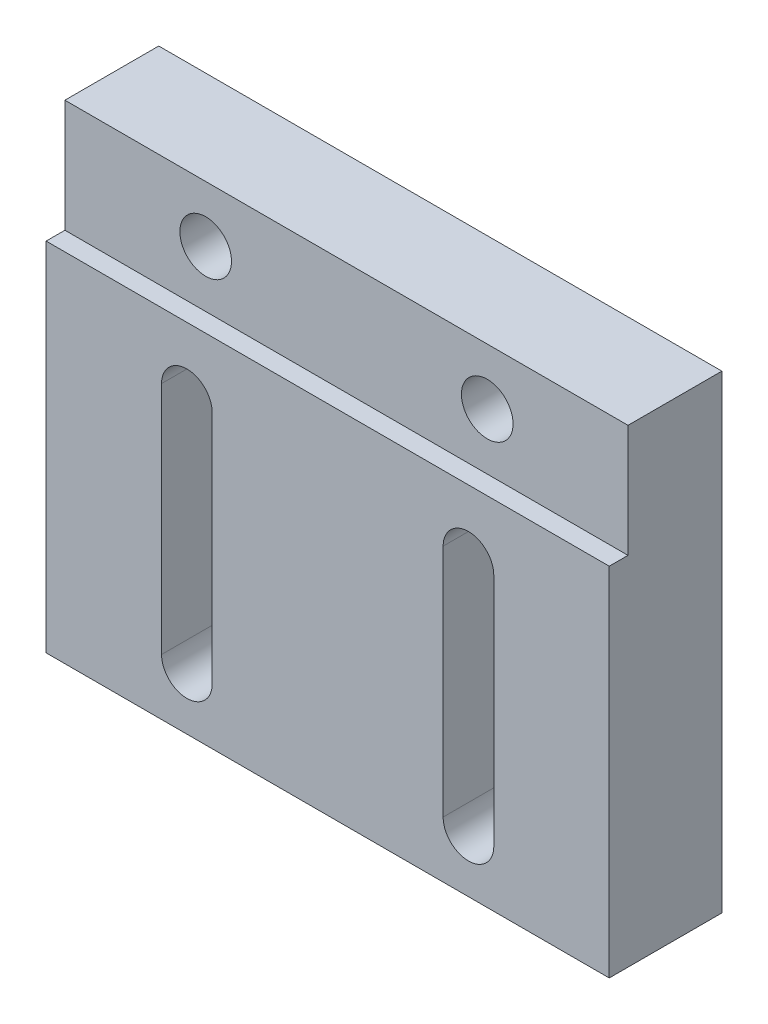
SolidWorks part; units mm, degrees
material "6061 合金"
ref_plane "前基準面" through (0, 0, 0) normal (0, 0, 1) x (1, 0, 0)
ref_plane "上基準面" through (0, 0, 0) normal (0, 1, 0) x (1, 0, 0)
ref_plane "右基準面" through (0, 0, 0) normal (1, 0, 0) x (0, 0, -1)
sketch "草图1" plane through (0, 0, 0) normal (0, 0, 1) x (1, 0, 0)
  line L1 (-30, 25) -> (30, 25)
  line L2 (-30, 25) -> (-30, -25)
  line L3 (-30, -25) -> (30, -25)
  line L4 (30, 25) -> (30, -25)
  line L5 (-30, 25) -> (30, -25) construction
  line L6 (-30, -25) -> (30, 25) construction
  point P0 (0, 0)
  dimension "D1" = 60
  dimension "D2" = 50
extrude "凸台-拉伸1" add sketch "草图1" along normal mid plane 12
sketch "草图2" plane through (0, 0, 6) normal (0, 0, 1) x (1, 0, 0)
  line L0 (30, -25) -> (30, 25) construction
  line L1 (-30, 25) -> (30, 25)
  line L2 (-30, 25) -> (-30, 13)
  line L3 (-30, 13) -> (30, 13)
  line L4 (30, 25) -> (30, 13)
  dimension "D1" = 12
extrude "切除-拉伸1" cut sketch "草图2" against normal blind 2
sketch "草图3" plane through (0, 0, 6) normal (0, 0, 1) x (1, 0, 0)
  line L0 (-15, -19) -> (-15, 6) construction
  line L1 (-17.7, -19) -> (-17.7, 6)
  line L2 (-12.3, -19) -> (-12.3, 6)
  line L3 (15, -19) -> (15, 6) construction
  line L4 (12.3, -19) -> (12.3, 6)
  line L5 (17.7, -19) -> (17.7, 6)
  line L6 (-15, -19) -> (15, -19) construction
  line L7 (0, -19) -> (0, -25) construction
  line L8 (-30, -25) -> (30, -25) construction
  arc A0 (-17.7, -19) -> (-12.3, -19) centre (-15, -19) ccw
  arc A1 (-12.3, 6) -> (-17.7, 6) centre (-15, 6) ccw
  arc A2 (12.3, -19) -> (17.7, -19) centre (15, -19) ccw
  arc A3 (17.7, 6) -> (12.3, 6) centre (15, 6) ccw
  point P2 (-15, -6.5)
  point P7 (15, -6.5)
  dimension "D1" = 2.7
  dimension "D2" = 6
  dimension "D3" = 30
  dimension "D4" = 25
extrude "切除-拉伸2" cut sketch "草图3" against normal through all
hole_wizard "M4 沉头孔1" positions "草图5" profile "草图4" counterbore size "M5" standard "ISO" end condition up to next
sketch "草图5" plane through (0, 0, -6) normal (0, 0, -1) x (-1, 0, 0)
  point P1 (-15, 19)
  point P4 (15, 19)
sketch "草图4" plane through (15, 19, -6) normal (1, 0, 0) x (0, 1, 0)
  line L0 (0, 0) -> (0, 10)
  line L1 (0, 10) -> (2.75, 10)
  line L3 (2.75, 10) -> (2.75, 5.4)
  line L4 (2.75, 5.4) -> (5, 5.4)
  line L5 (5, 5.4) -> (5, 0)
  line L7 (5, 0) -> (0, 0)
  line L11 (0, -6.35) -> (0, 107.95) construction
  dimension "通孔孔直径" = 5.5
  dimension "通孔孔深度" = 10
  dimension "柱形沉头孔直径" = 10
  dimension "柱形沉头孔深度" = 5.4
